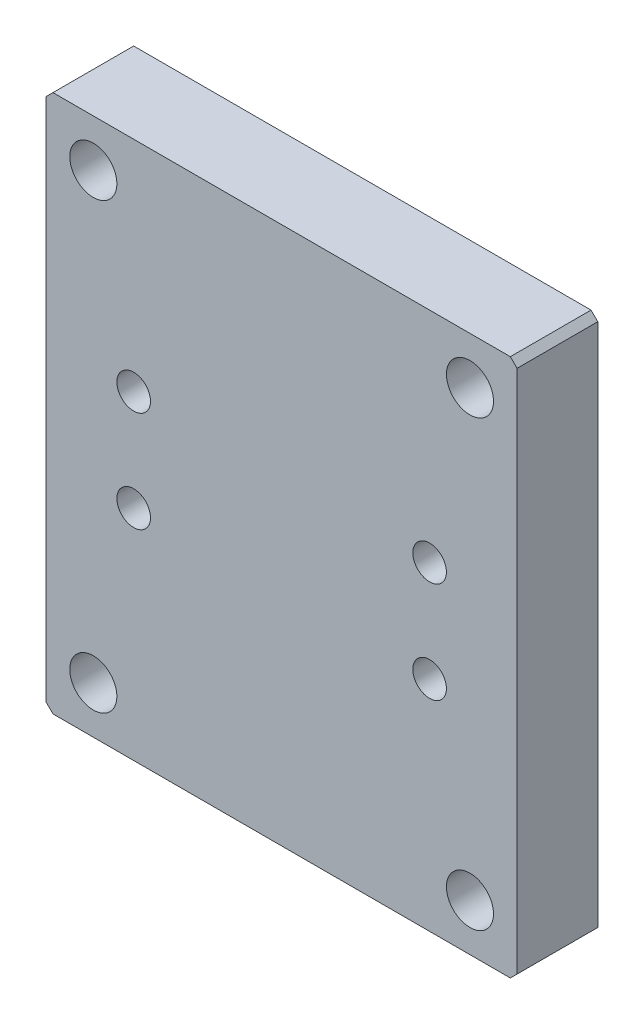
SolidWorks part; units mm, degrees
ref_plane "前视" through (0, 0, 0) normal (0, 0, 1) x (1, 0, 0)
ref_plane "上视" through (0, 0, 0) normal (0, 1, 0) x (1, 0, 0)
ref_plane "右视" through (0, 0, 0) normal (1, 0, 0) x (0, 0, -1)
sketch "草图1" plane through (0, 0, 0) normal (0, 0, 1) x (1, 0, 0)
  line L1 (0, 0) -> (70, 0)
  line L2 (0, 0) -> (0, -80)
  line L3 (0, -80) -> (70, -80)
  line L4 (70, 0) -> (70, -80)
  dimension "D1" = 70
  dimension "D2" = 80
extrude "凸台-拉伸1" add sketch "草图1" along normal blind 12
chamfer "倒角1" distance 1 angle 45 4 edges at (0, -80, 6) (70, -80, 6) (70, 0, 6) (0, 0, 6)
sketch "草图2" plane through (0, 0, 12) normal (0, 0, 1) x (1, 0, 0)
  line L0 (17.5, -5) -> (52.5, -5) construction
  line L1 (17.5, -2.5) -> (52.5, -2.5)
  line L2 (17.5, -7.5) -> (52.5, -7.5)
  line L3 (35, -2.5) -> (35, 0) construction
  line L4 (69, 0) -> (1, 0) construction
  arc A0 (17.5, -2.5) -> (17.5, -7.5) centre (17.5, -5) ccw
  arc A1 (52.5, -7.5) -> (52.5, -2.5) centre (52.5, -5) ccw
  point P2 (35, -5)
  dimension "D1" = 5
  dimension "D2" = 2.5
  dimension "D3" = 35
extrude "切除-拉伸1" [suppressed] cut sketch "草图2" against normal blind 2.5
pattern_linear "阵列(线性)1" [suppressed] count 8 spacing 10
hole_wizard "Ø7.0 (7) 直径孔1" positions "草图4" profile "草图3" hole size "Ø7.0" standard "ISO" end condition through all
sketch "草图4" plane through (0, 0, 0) normal (0, 0, -1) x (-1, 0, 0)
  line L1 (-7, -73) -> (-63, -73)
  line L2 (-7, -73) -> (-7, -7)
  line L3 (-7, -7) -> (-63, -7)
  line L4 (-63, -73) -> (-63, -7)
  line L5 (-35, -73) -> (-35, -80) construction
  line L6 (-1, -80) -> (-69, -80) construction
  line L8 (-63, -40) -> (-70, -40) construction
  line L9 (-70, -79) -> (-70, -1) construction
  point P0 (-7, -73)
  point P2 (-7, -7)
  point P4 (-63, -73)
  point P6 (-63, -7)
  dimension "D1" = 7
  dimension "D2" = 7
sketch "草图3" plane through (7, -73, 0) normal (1, 0, 0) x (0, 1, 0)
  line L0 (0, 0) -> (0, 12)
  line L1 (0, 12) -> (3.5, 12)
  line L2 (3.5, 12) -> (3.5, 0)
  line L5 (3.5, 0) -> (0, 0)
  line L11 (0, -6.35) -> (0, 107.95) construction
  dimension "通孔孔直径" = 7
  dimension "通孔孔深度" = 12
hole_wizard "M6 螺纹孔1" positions "草图6" profile "草图5" tap size "M6" standard "GB" end condition through all
sketch "草图6" plane through (0, 0, 0) normal (0, 0, -1) x (-1, 0, 0)
  point P0 (-57, -32.5)
  point P3 (-57, -47.5)
  point P6 (-13, -47.5)
  point P9 (-13, -32.5)
sketch "草图5" plane through (57, -32.5, 0) normal (1, 0, 0) x (0, 1, 0)
  line L0 (0, 0) -> (0, 12)
  line L1 (0, 12) -> (2.5, 12)
  line L2 (2.5, 12) -> (2.5, 0)
  line L5 (2.5, 0) -> (0, 0)
  line L11 (0, -6.35) -> (0, 107.95) construction
  dimension "通孔螺纹孔钻头直径" = 5
  dimension "通孔螺纹孔钻头深度" = 12
cosmetic thread "孔螺蚊线5" parameters "D2"=6
cosmetic thread "孔螺蚊线6" parameters "D2"=6
cosmetic thread "孔螺蚊线7" parameters "D2"=6
cosmetic thread "孔螺蚊线8" parameters "D2"=6
